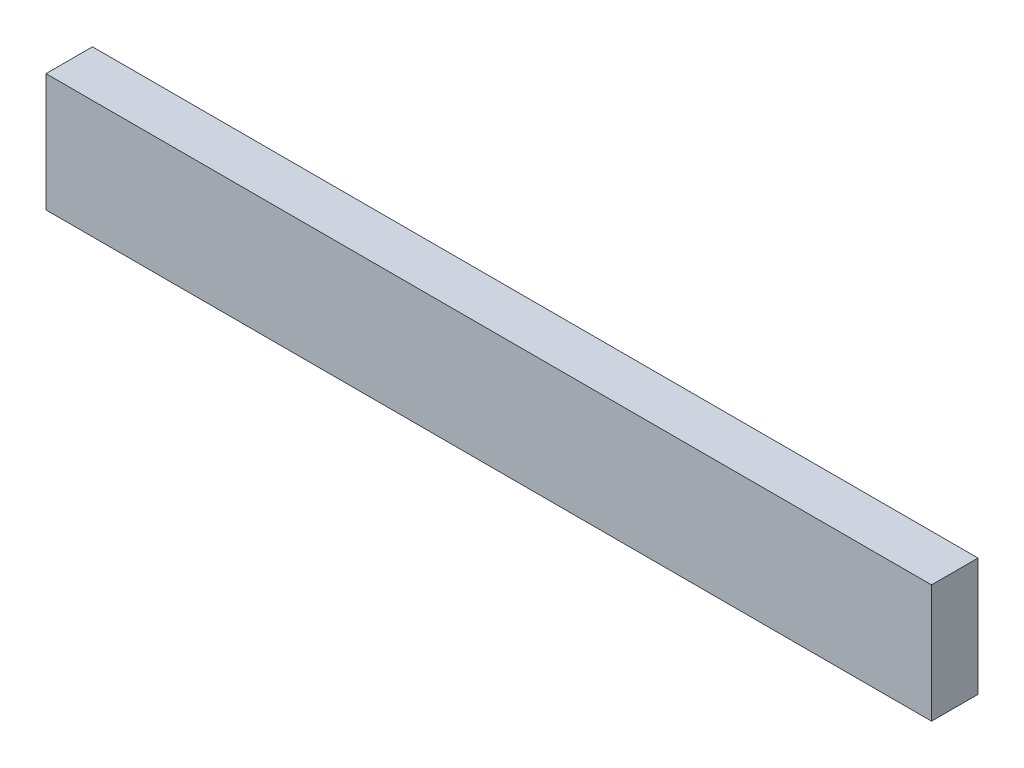
from build123d import *

# Parameters (mm, degrees)
SKETCH1_W           = 190.5
SKETCH1_H           = 25.4
BOSS_EXTRUDE1_DEPTH = 5


with BuildPart() as part:
    # Sketch1 → Boss-Extrude1 (new, symmetric)
    with BuildSketch(Plane.XY):
        Rectangle(SKETCH1_W, SKETCH1_H)
    extrude(amount=BOSS_EXTRUDE1_DEPTH, both=True)


solid = part.part
